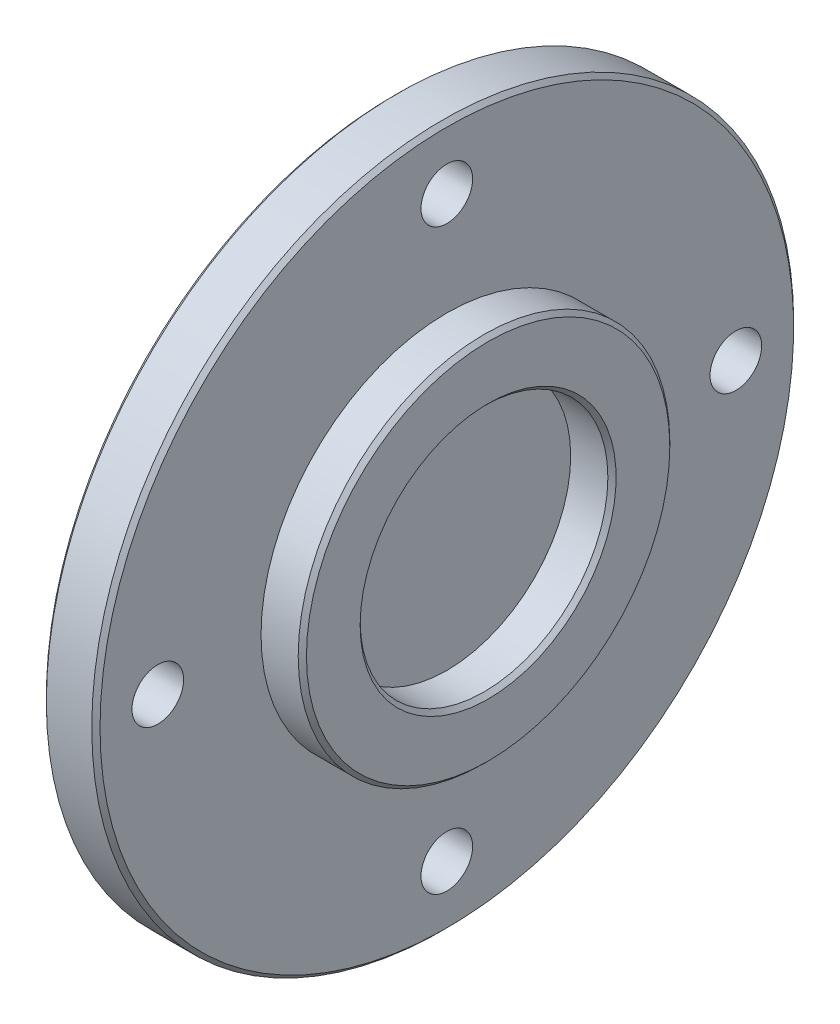
from build123d import *

# Parameters (mm, degrees)
SKETCH_2_R               = 6.25
CUT_EXTRUDE_1_DEPTH      = 123.388724971
PATTERN_CIRCULAR_1_COUNT = 4
CHAMFER_1_SIZE           = 1


with BuildPart() as part:
    # 草图1 → 旋转1 (revolve)
    with BuildSketch(Plane.XY, mode=Mode.PRIVATE) as revolve_1_sk:
        Polygon((0, 0), (0, 85), (13, 85), (13, 45), (23, 45), (23, 30), (13, 30), (13, 0), align=None)
    revolve(revolve_1_sk.sketch.rotate(Axis((0, 0, 0), (1, 0, 0)), 90), axis=Axis((0, 0, 0), (1, 0, 0)))

    # 草图2 → 切除-拉伸1 (cut, through all)
    with BuildSketch(Plane.ZY):
        with Locations((0, 70)):
            Circle(SKETCH_2_R)
    cut_extrude_1 = extrude(amount=-CUT_EXTRUDE_1_DEPTH, mode=Mode.SUBTRACT)

    # 阵列(圆周)1: 切除-拉伸1 ×4 about axis
    pattern_circular_1_axis = Axis((0, 0, 0), (1, 0, 0))
    for i in range(1, PATTERN_CIRCULAR_1_COUNT):
        add(cut_extrude_1.rotate(pattern_circular_1_axis, i * 360 / PATTERN_CIRCULAR_1_COUNT), mode=Mode.SUBTRACT)

    # 倒角1
    chamfer_1_edges = [part.edges().sort_by_distance(p)[0] for p in [
        (23, 0, -30),
        (23, 0, -45),
        (13, 0, -85),
        (0, 0, -85),
    ]]
    chamfer(chamfer_1_edges, length=CHAMFER_1_SIZE)


solid = part.part
